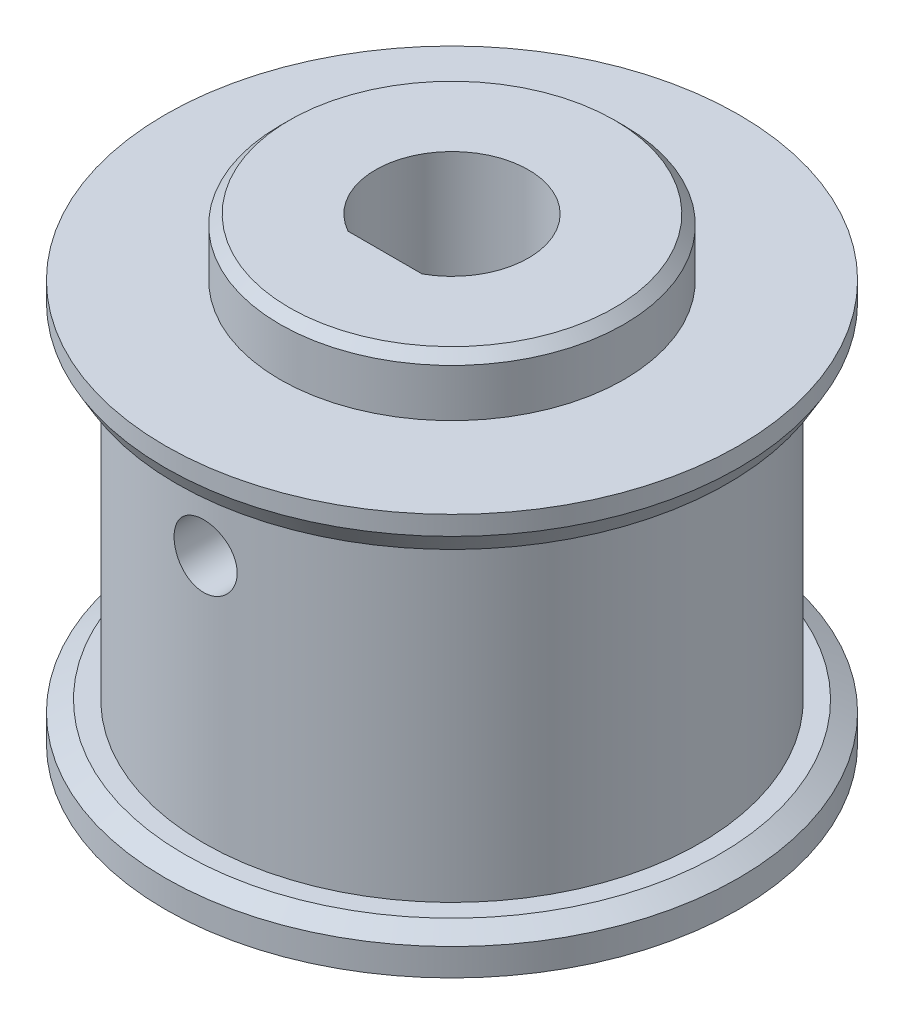
SolidWorks part; units mm, degrees
material "6061 合金"
ref_plane "前视基准面" through (0, 0, 0) normal (0, 0, 1) x (1, 0, 0)
ref_plane "上视基准面" through (0, 0, 0) normal (0, 1, 0) x (1, 0, 0)
ref_plane "右视基准面" through (0, 0, 0) normal (1, 0, 0) x (0, 0, -1)
sketch "草图1" plane through (0, 0, 0) normal (0, 0, 1) x (1, 0, 0)
  line L0 (0, 0) -> (0, 32.2299) construction
  line L1 (4, 0) -> (4, 21)
  line L2 (4, 21) -> (15, 21)
  line L3 (15, 21) -> (15, 19)
  line L4 (15, 19) -> (12.99, 19)
  line L5 (12.99, 19) -> (12.99, 2)
  line L6 (12.99, 2) -> (15, 2)
  line L7 (15, 2) -> (15, 0)
  line L8 (15, 0) -> (4, 0)
  dimension "D1" = 2
  dimension "D2" = 2
  dimension "D3" = 8
  dimension "D4" = 25.98
  dimension "D5" = 30
  dimension "D6" = 21
revolve "旋转1" add sketch "草图1" angle 360 about L0
sketch "草图5" plane through (0, 0, 0) normal (0, -1, 0) x (1, 0, 0)
  circle A0 centre (0, 0) radius 20.5663
extrude "切除-拉伸1" cut sketch "草图5" against normal blind 0.5
sketch "草图6" plane through (0, 21, 0) normal (0, 1, 0) x (1, 0, 0)
  circle A0 centre (0, 0) radius 21.5283
extrude "切除-拉伸2" cut sketch "草图6" against normal blind 0.5
sketch "草图7" plane through (0, 20.5, 0) normal (0, 1, 0) x (1, 0, 0)
  circle A0 centre (0, 0) radius 4 construction
  circle A1 centre (0, 0) radius 4
  circle A2 centre (0, 0) radius 8.5
  dimension "D1" = 17
extrude "凸台-拉伸1" add sketch "草图7" along normal blind 11
sketch "草图10" plane through (0, 20.5, 0) normal (0, 1, 0) x (1, 0, 0)
  circle A1 centre (0, 0) radius 15
  circle A2 centre (0, 0) radius 15
  dimension "D1" = 0
extrude "切除-拉伸3" cut sketch "草图10" along normal blind 15
sketch "草图11" plane through (0, 20.5, 0) normal (0, 1, 0) x (1, 0, 0)
  circle A0 centre (0, 0) radius 4 construction
  circle A1 centre (0, 0) radius 15
  circle A2 centre (0, 0) radius 15
  circle A3 centre (0, 0) radius 4
  dimension "D1" = 0
extrude "凸台-拉伸2" add sketch "草图11" along normal blind 0.5
sketch "草图12" plane through (0, 0.5, 0) normal (0, -1, 0) x (1, 0, 0)
  circle A0 centre (0, 0) radius 4 construction
  circle A1 centre (0, 0) radius 15
  circle A2 centre (0, 0) radius 15
  circle A3 centre (0, 0) radius 4
  dimension "D1" = 0
extrude "凸台-拉伸3" add sketch "草图12" along normal blind 0.5
sketch "草图14" plane through (0, 21, 0) normal (0, 1, 0) x (1, 0, 0)
  circle A0 centre (0, 0) radius 4 construction
  circle A1 centre (0, 0) radius 4
  circle A2 centre (0, 0) radius 7
  dimension "D1" = 14
extrude "凸台-拉伸5" add sketch "草图14" along normal blind 8
sketch "草图17" plane through (0, 21, 0) normal (0, 1, 0) x (1, 0, 0)
  circle A0 centre (0, 0) radius 17.2152
extrude "切除-拉伸4" cut sketch "草图17" along normal through all
sketch "草图18" plane through (0, 21, 0) normal (0, 1, 0) x (1, 0, 0)
  circle A0 centre (0, 0) radius 4 construction
  circle A1 centre (0, 0) radius 4
  circle A2 centre (0, 0) radius 9
  dimension "D1" = 18
extrude "凸台-拉伸6" add sketch "草图18" along normal blind 8
chamfer "倒角1" distance 1 angle 30 1 edges at (0, 19, -15)
chamfer "倒角2" distance 1 angle 30 1 edges at (0, 2, -15)
chamfer "倒角3" distance 0.5 angle 45 1 edges at (0, 29, 9)
sketch "草图21" plane through (0, 29, 0) normal (0, 1, 0) x (1, 0, 0)
  circle A0 centre (0, 0) radius 7
  dimension "D1" = 14
extrude "切除-拉伸5" [suppressed] cut sketch "草图21" against normal blind 52
sketch "草图22" plane through (0, 29, 0) normal (0, 1, 0) x (1, 0, 0)
  circle A0 centre (0, 0) radius 10.406
extrude "切除-拉伸6" cut sketch "草图22" against normal blind 5
sketch "草图24" plane through (0, 0, 0) normal (0, -1, 0) x (1, 0, 0)
  line L1 (-3.1991, 4.766) -> (3.851, 4.766)
  line L2 (-3.1991, 4.766) -> (-3.1991, 3.5)
  line L3 (-3.1991, 3.5) -> (3.851, 3.5)
  line L4 (3.851, 4.766) -> (3.851, 3.5)
  dimension "D1" = 3.5
extrude "凸台-拉伸7" add sketch "草图24" against normal up to surface (24 mm away) up to face at (0, 24, 4)
hole_wizard "M4 螺纹孔1" positions "草图20" profile "草图19" tap size "M4" standard "GB"
sketch "草图20" plane through (0, 0, 0) normal (0, 0, 1) x (1, 0, 0)
  line L1 (9, 24) -> (-9, 24) construction
  point P0 (0, 15)
  dimension "D2" = 9
sketch "草图19" plane through (0, 15, 0) normal (1, 0, 0) x (0, 1, 0)
  line L0 (0, 0) -> (0, 15)
  line L1 (0, 15) -> (1.65, 15)
  line L2 (1.65, 15) -> (1.65, 0)
  line L5 (1.65, 0) -> (0, 0)
  line L11 (0, -6.35) -> (0, 107.95) construction
  dimension "通孔螺纹孔钻头直径" = 3.3
  dimension "通孔螺纹孔钻头深度" = 15
cosmetic thread "孔螺蚊线1" parameters "D2"=4
pattern_circular "阵列(圆周)1" count 2 every 90 of "M4 螺纹孔1"
chamfer "倒角4" distance 0.5 angle 45 1 edges at (0, 24, 9)
